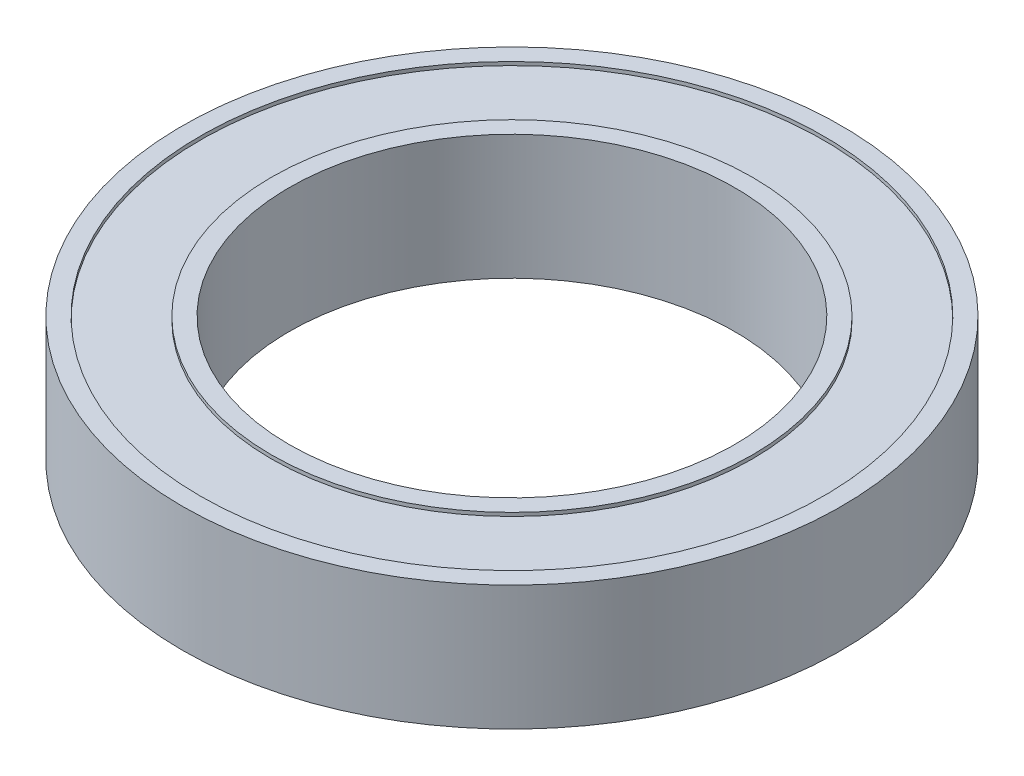
SolidWorks part; units mm, degrees
material "AISI 304"
ref_plane "Front Plane" through (0, 0, 0) normal (0, 0, 1) x (1, 0, 0)
ref_plane "Top Plane" through (0, 0, 0) normal (0, 1, 0) x (1, 0, 0)
ref_plane "Right Plane" through (0, 0, 0) normal (1, 0, 0) x (0, 0, -1)
sketch "Sketch1" plane through (0, 0, 0) normal (0, 1, 0) x (1, 0, 0)
  circle A0 centre (0, 0) radius 18.5
  circle A1 centre (0, 0) radius 12.5
  dimension "D1" = 25
  dimension "D2" = 37
extrude "Boss-Extrude1" add sketch "Sketch1" along normal blind 7
sketch "Sketch2" plane through (0, 7, 0) normal (0, 1, 0) x (1, 0, 0)
  circle A0 centre (0, 0) radius 13.5
  circle A1 centre (0, 0) radius 17.5
  dimension "D1" = 27
  dimension "D2" = 35
extrude "Cut-Extrude1" cut sketch "Sketch2" against normal blind 0.2
sketch "Sketch3" plane through (0, 0, 0) normal (0, -1, 0) x (1, 0, 0)
  circle A0 centre (0, 0) radius 13.5
  circle A1 centre (0, 0) radius 17.5
  dimension "D1" = 27
  dimension "D2" = 35
extrude "Cut-Extrude2" cut sketch "Sketch3" against normal blind 0.2
